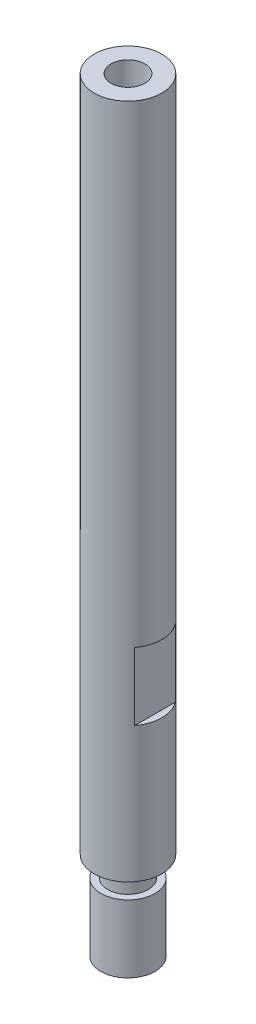
from build123d import *

# Parameters (mm, degrees)
CUT_EXTRUDE1_DEPTH      = 100.081673268
CUT_EXTRUDE1_DEPTH_BACK = 100.081673268
SKETCH2_W               = 1
SKETCH2_H               = 10
M6_TAPPED_HOLE1_D       = 5
M6_TAPPED_HOLE1_DEPTH   = 12
M6_TAPPED_HOLE1_TIP     = 1.502151548


with BuildPart() as part:
    # Sketch1 → Revolve1 (revolve)
    with BuildSketch(Plane.XY):
        Polygon((0, 14.170965918), (0, -98.829034082), (-4, -98.829034082), (-4, -88.829034082), (-3, -88.829034082), (-3, -85.829034082), (-5, -85.829034082), (-5, 14.170965918), align=None)
    revolve(axis=Axis((0, 14.170965918, 0), (0, -1, 0)))

    # Sketch2 → Cut-Extrude1 (cut, two sides: drawn at the far end of the back side and taken through both)
    with BuildSketch(Plane.XY.offset(-CUT_EXTRUDE1_DEPTH_BACK)):
        with Locations((-4.5, -60.829034082)):
            Rectangle(SKETCH2_W, SKETCH2_H)
        with Locations((4.5, -60.829034082)):
            Rectangle(SKETCH2_W, SKETCH2_H)
    extrude(amount=CUT_EXTRUDE1_DEPTH + CUT_EXTRUDE1_DEPTH_BACK, mode=Mode.SUBTRACT)

    # M6 Tapped Hole1
    with Locations(Plane(origin=(0, 14.170965918, 0), x_dir=(1, 0, 0), z_dir=(0, 1, 0))):
        with Locations((0, 0)):
            Hole(M6_TAPPED_HOLE1_D / 2, depth=M6_TAPPED_HOLE1_DEPTH)
            with Locations((0, 0, -(M6_TAPPED_HOLE1_DEPTH + M6_TAPPED_HOLE1_TIP / 2))):  # 118° drill point
                Cone(0, M6_TAPPED_HOLE1_D / 2, M6_TAPPED_HOLE1_TIP, mode=Mode.SUBTRACT)


solid = part.part
